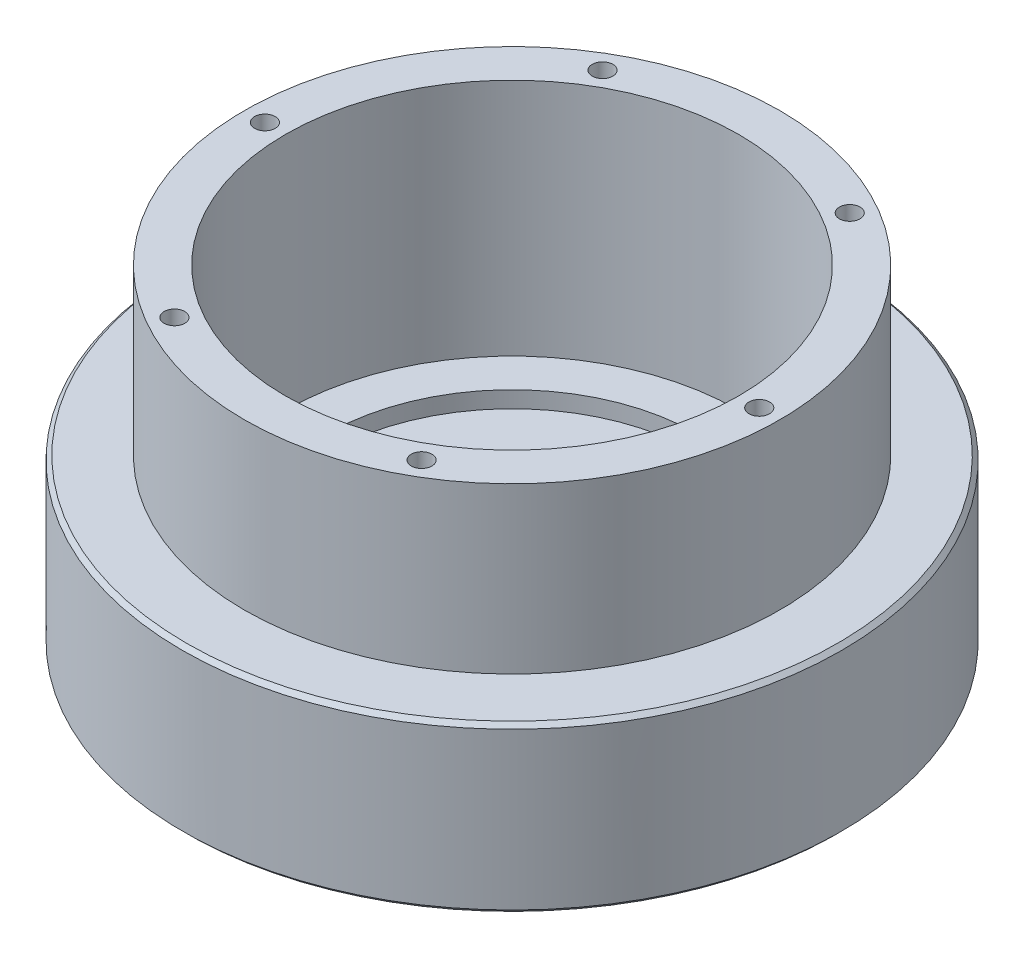
SolidWorks part; units mm, degrees
ref_plane "Front Plane" through (0, 0, 0) normal (0, 0, 1) x (1, 0, 0)
ref_plane "Top Plane" through (0, 0, 0) normal (0, 1, 0) x (1, 0, 0)
ref_plane "Right Plane" through (0, 0, 0) normal (1, 0, 0) x (0, 0, -1)
sketch "Sketch1" plane through (0, 0, 0) normal (0, 0, 1) x (1, 0, 0)
  line L0 (0, 0) -> (0, 25741.0304) construction
  line L1 (0, 0) -> (40, 0)
  line L2 (40, 0) -> (40, 20)
  line L3 (40, 20) -> (32.5, 20)
  line L4 (32.5, 20) -> (32.5, 40)
  line L5 (32.5, 40) -> (0, 40)
  line L8 (0, 40) -> (0, 0)
  dimension "D1" = 80
  dimension "D2" = 65
  dimension "D3" = 40
  dimension "D4" = 20
revolve "Revolve1" add sketch "Sketch1" angle 360 about L0
sketch "Sketch2" plane through (0, 0, 0) normal (0, 0, 1) x (1, 0, 0)
  line L0 (0, 0) -> (0, 50000) construction
  line L1 (0, 40) -> (27.5, 40)
  line L2 (32.5, 40) -> (-32.5, 40) construction
  line L3 (27.5, 40) -> (27.5, 11)
  line L4 (27.5, 11) -> (22.5, 11)
  line L5 (22.5, 11) -> (22.5, 9)
  line L6 (22.5, 9) -> (16, 9)
  line L7 (16, 9) -> (16, 0)
  line L8 (-40, 0) -> (40, 0) construction
  line L9 (16, 0) -> (0, 0)
  line L10 (0, 0) -> (0, 40)
  dimension "D1" = 55
  dimension "D2" = 45
  dimension "D3" = 32
  dimension "D4" = 9
  dimension "D5" = 2
revolve "Cut-Revolve1" cut sketch "Sketch2" angle 360 about L0
hole_wizard "M3 Tapped Hole1" positions "Sketch3" profile "Sketch4" tap size "M3" standard "GB"
sketch "Sketch3" plane through (0, 40, 0) normal (0, 1, 0) x (1, 0, 0)
  circle A0 centre (0, 0) radius 30 construction
  point P0 (-30, 0)
  point P14 (-15, 25.9808)
  point P15 (15, 25.9808)
  point P16 (30, 0)
  point P17 (15, -25.9808)
  point P18 (-15, -25.9808)
  point P19 (0, 0)
  dimension "D1" = 60
  dimension "D2" = 6
sketch "Sketch4" plane through (-30, 40, 0) normal (1, 0, 0) x (0, 0, 1)
  line L0 (0, 0) -> (0, 8.2511)
  line L1 (0, 8.2511) -> (1.25, 7.5)
  line L2 (1.25, 7.5) -> (1.25, 0)
  line L5 (1.25, 0) -> (0, 0)
  line L10 (0, 8.2511) -> (-1.25, 7.5) construction
  line L11 (0, -6.35) -> (0, 107.95) construction
  dimension "螺纹孔钻头直径" = 2.5
  dimension "螺纹孔钻头深度" = 7.5
  dimension "导头角度" = 118
cosmetic thread "Cosmetic thread 1" parameters "D1"=6, "D2"=3
cosmetic thread "Cosmetic thread 2" parameters "D1"=6, "D2"=3
cosmetic thread "Cosmetic thread 3" parameters "D1"=6, "D2"=3
cosmetic thread "Cosmetic thread 4" parameters "D1"=6, "D2"=3
cosmetic thread "Cosmetic thread 5" parameters "D1"=6, "D2"=3
cosmetic thread "Cosmetic thread 6" parameters "D1"=6, "D2"=3
chamfer "Chamfer1" distance 0.5 angle 45
hole_wizard "M4 Tapped Hole1" positions "Sketch5" profile "Sketch6" tap size "M4" standard "GB"
sketch "Sketch5" plane through (0, 0, 0) normal (0, -1, 0) x (-1, 0, 0)
  point P0 (18.8145, 29.4123)
sketch "Sketch6" plane through (-18.8145, 0, -29.4123) normal (1, 0, 0) x (0, 0, -1)
  line L0 (0, 0) -> (0, 11.0914)
  line L1 (0, 11.0914) -> (1.65, 10.1)
  line L2 (1.65, 10.1) -> (1.65, 0)
  line L5 (1.65, 0) -> (0, 0)
  line L10 (0, 11.0914) -> (-1.65, 10.1) construction
  line L11 (0, -6.35) -> (0, 107.95) construction
  dimension "螺纹孔钻头直径" = 3.3
  dimension "螺纹孔钻头深度" = 10.1
  dimension "导头角度" = 118
cosmetic thread "Cosmetic thread 7" parameters "D1"=8, "D2"=4
hole_wizard "M3 Tapped Hole2" positions "Sketch7" profile "Sketch8" tap size "M3" standard "GB"
sketch "Sketch7" plane through (0, 0, 0) normal (0, -1, 0) x (-1, 0, 0)
  point P0 (-34.3349, 15.4697)
  point P3 (-25.8349, 0.7473)
sketch "Sketch8" plane through (34.3349, 0, -15.4697) normal (1, 0, 0) x (0, 0, -1)
  line L0 (0, 0) -> (0, 8.2511)
  line L1 (0, 8.2511) -> (1.25, 7.5)
  line L2 (1.25, 7.5) -> (1.25, 0)
  line L5 (1.25, 0) -> (0, 0)
  line L10 (0, 8.2511) -> (-1.25, 7.5) construction
  line L11 (0, -6.35) -> (0, 107.95) construction
  dimension "螺纹孔钻头直径" = 2.5
  dimension "螺纹孔钻头深度" = 7.5
  dimension "导头角度" = 118
cosmetic thread "Cosmetic thread 8" parameters "D1"=6, "D2"=3
cosmetic thread "Cosmetic thread 9" parameters "D1"=6, "D2"=3
hole_wizard "M3 Tapped Hole3" positions "Sketch9" profile "Sketch10" tap size "M3" standard "GB"
sketch "Sketch9" plane through (0, 0, 0) normal (0, -1, 0) x (-1, 0, 0)
  point P0 (4.9892, 28.3585)
  point P3 (-12.3313, 18.3585)
  point P6 (-29.6518, 8.3585)
sketch "Sketch10" plane through (-4.9892, 0, -28.3585) normal (1, 0, 0) x (0, 0, -1)
  line L0 (0, 0) -> (0, 8.2511)
  line L1 (0, 8.2511) -> (1.25, 7.5)
  line L2 (1.25, 7.5) -> (1.25, 0)
  line L5 (1.25, 0) -> (0, 0)
  line L10 (0, 8.2511) -> (-1.25, 7.5) construction
  line L11 (0, -6.35) -> (0, 107.95) construction
  dimension "螺纹孔钻头直径" = 2.5
  dimension "螺纹孔钻头深度" = 7.5
  dimension "导头角度" = 118
cosmetic thread "Cosmetic thread 10" parameters "D1"=6, "D2"=3
cosmetic thread "Cosmetic thread 11" parameters "D1"=6, "D2"=3
cosmetic thread "Cosmetic thread 12" parameters "D1"=6, "D2"=3
hole_wizard "M4 Tapped Hole2" positions "Sketch11" profile "Sketch12" tap size "M4" standard "GB"
sketch "Sketch11" plane through (0, 0, 0) normal (0, -1, 0) x (-1, 0, 0)
  point P0 (22.9103, -19.6817)
  point P3 (5.5897, -29.6817)
sketch "Sketch12" plane through (-22.9103, 0, 19.6817) normal (1, 0, 0) x (0, 0, -1)
  line L0 (0, 0) -> (0, 11.0914)
  line L1 (0, 11.0914) -> (1.65, 10.1)
  line L2 (1.65, 10.1) -> (1.65, 0)
  line L5 (1.65, 0) -> (0, 0)
  line L10 (0, 11.0914) -> (-1.65, 10.1) construction
  line L11 (0, -6.35) -> (0, 107.95) construction
  dimension "螺纹孔钻头直径" = 3.3
  dimension "螺纹孔钻头深度" = 10.1
  dimension "导头角度" = 118
cosmetic thread "Cosmetic thread 13" parameters "D1"=8, "D2"=4
cosmetic thread "Cosmetic thread 14" parameters "D1"=8, "D2"=4
